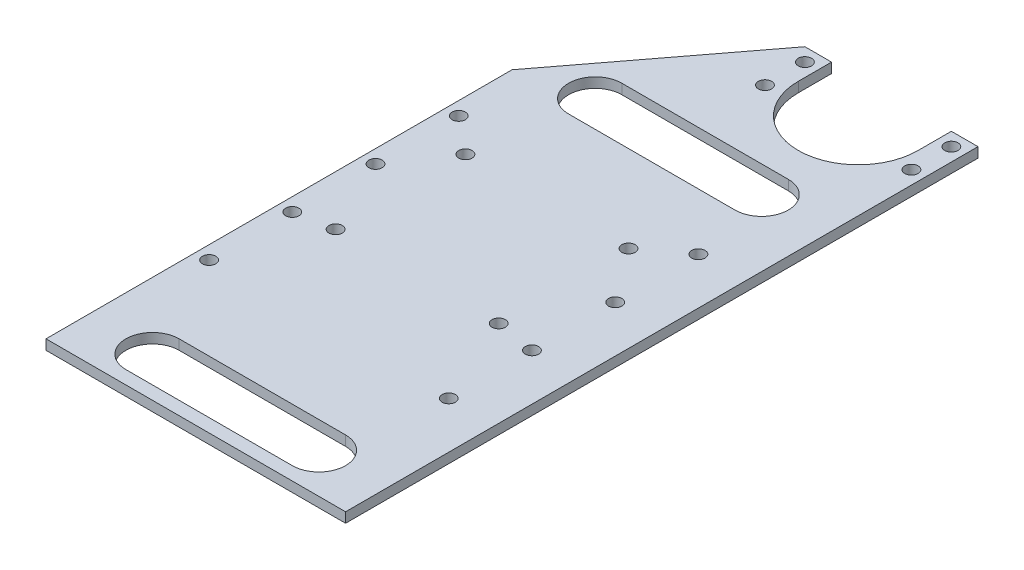
SolidWorks part; units mm, degrees
ref_plane "Front Plane" through (0, 0, 0) normal (0, 0, 1) x (1, 0, 0)
ref_plane "Top Plane" through (0, 0, 0) normal (0, 1, 0) x (1, 0, 0)
ref_plane "Right Plane" through (0, 0, 0) normal (1, 0, 0) x (0, 0, -1)
sketch "Sketch1" plane through (0, 0, 0) normal (0, 1, 0) x (1, 0, 0)
  line L0 (0, 123.2692) -> (0, -155.9615) construction
  line L2 (-12, -7.2619) -> (40, -7.2619)
  line L5 (40, -197.2619) -> (-50, -197.2619)
  line L13 (-50, -57.2619) -> (-50, -197.2619)
  line L14 (-12, -7.2619) -> (-50, -57.2619)
  line L15 (40, -197.2619) -> (40, -7.2619)
  point P13 (0, -7.2619)
  dimension "D5" = 40
  dimension "D1" = 50
  dimension "D2" = 50
  dimension "D3" = 190
  dimension "D4" = 52
extrude "Boss-Extrude1" add sketch "Sketch1" along normal blind 3
sketch "Sketch2" plane through (0, 3, 0) normal (0, 1, 0) x (1, 0, 0)
  line L0 (-5, -7.2619) -> (-5, -197.2619) construction
  line L1 (36, -23.2619) -> (36, -11.2619) construction
  line L2 (-50, -197.2619) -> (40, -197.2619) construction
  line L3 (-46, -77.2619) -> (-46, -152.2619) construction
  line L5 (-50, -57.2619) -> (-50, -197.2619) construction
  line L6 (40, -197.2619) -> (40, -7.2619) construction
  line L7 (20, -185.2619) -> (-30, -185.2619) construction
  line L20 (20, -193.2619) -> (-30, -193.2619)
  line L25 (-50, -197.2619) -> (40, -197.2619) construction
  line L32 (40, -7.2619) -> (-12, -7.2619) construction
  line L33 (-8, -23.2619) -> (-8, -11.2619) construction
  line L34 (-8, -17.2619) -> (14, -17.2619) construction
  line L35 (26, -77.2619) -> (26, -152.2619) construction
  line L36 (20, -52.2619) -> (-30, -52.2619) construction
  line L37 (20, -60.2619) -> (-30, -60.2619)
  line L38 (20, -44.2619) -> (-30, -44.2619)
  line L39 (14, -7.2619) -> (14, -30.7814) construction
  line L40 (40, -7.2619) -> (-12, -7.2619) construction
  line L46 (32, -17.2619) -> (32, -7.2619)
  line L47 (-35, -86.2619) -> (-35, -125.2619) construction
  line L50 (-4, -17.2619) -> (-4, -7.2619)
  line L51 (-4, -7.2619) -> (32, -7.2619)
  line L52 (20, -177.2619) -> (-30, -177.2619)
  line L53 (-50, -197.2619) -> (40, -197.2619) construction
  line L54 (40, -7.2619) -> (-12, -7.2619) construction
  line L55 (-12, -7.2619) -> (40, -7.2619) construction
  line L56 (14, -86.2619) -> (14, -125.2619) construction
  circle A47 centre (-46, -152.2619) radius 2
  circle A48 centre (-46, -77.2619) radius 2
  circle A52 centre (-46, -127.2619) radius 2
  circle A53 centre (-46, -102.2619) radius 2
  circle A55 centre (45.2788, -192.2619) radius 1.5
  circle A62 centre (-8, -11.2619) radius 2
  circle A63 centre (-8, -23.2619) radius 2
  circle A66 centre (26, -152.2619) radius 2
  circle A67 centre (26, -102.2619) radius 2
  circle A68 centre (26, -127.2619) radius 2
  circle A69 centre (26, -77.2619) radius 2
  arc A70 (20, -60.2619) -> (20, -44.2619) centre (20, -52.2619) ccw
  arc A71 (-30, -44.2619) -> (-30, -60.2619) centre (-30, -52.2619) ccw
  arc A72 (-4, -17.2619) -> (32, -17.2619) centre (14, -17.2619) ccw
  circle A73 centre (36, -23.2619) radius 2
  circle A74 centre (36, -11.2619) radius 2
  arc A75 (20, -193.2619) -> (20, -177.2619) centre (20, -185.2619) ccw
  arc A76 (-30, -177.2619) -> (-30, -193.2619) centre (-30, -185.2619) ccw
  circle A77 centre (-35, -86.2619) radius 2
  circle A78 centre (-35, -125.2619) radius 2
  circle A79 centre (14, -86.2619) radius 2
  circle A80 centre (14, -125.2619) radius 2
  point P38 (-5, -185.2619)
  point P47 (-5, -52.2619)
  dimension "D3" = 4
  dimension "D6" = 25
  dimension "D7" = 25
  dimension "D8" = 45
  dimension "D14" = 36
  dimension "D17" = 60
  dimension "D18" = 25
  dimension "D19" = 8
  dimension "D25" = 15
  dimension "D27" = 49
  dimension "D22" = 50
  dimension "D23" = 50
  dimension "D24" = 12
  dimension "D15" = 12
  dimension "D5" = 25
  dimension "D13" = 4
  dimension "D9" = 4
  dimension "D21" = 8
  dimension "D4" = 39
  dimension "D10" = 60
  dimension "D11" = 5
  dimension "D12" = 25
  dimension "D16" = 25
  dimension "D20" = 72
  dimension "D26" = 48
extrude "Cut-Extrude1" cut sketch "Sketch2" against normal up to surface (3 mm away)
